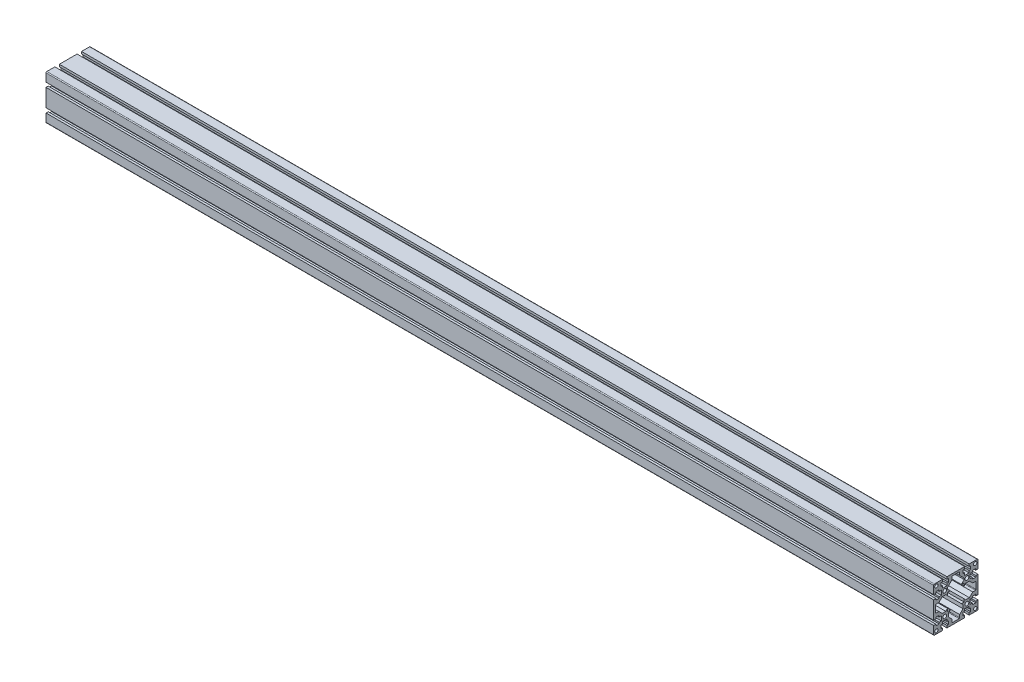
SolidWorks part; units mm, degrees
ref_plane "Front Plane" through (0, 0, 0) normal (0, 0, 1) x (1, 0, 0)
ref_plane "Top Plane" through (0, 0, 0) normal (0, 1, 0) x (1, 0, 0)
ref_plane "Right Plane" through (0, 0, 0) normal (1, 0, 0) x (0, 0, -1)
sketch "草图1" plane through (0, 0, 0) normal (0, 0, 1) x (1, 0, 0)
  line L0 (-530.3448, 0) -> (1069.6552, 0)
  dimension "D1" = 1600
other "Aluminum profile 80 X 80G X R1.5(1)"
ref_plane "Plane2" through (-530.3448, 0, 0) normal (1, 0, 0) x (0, 1, 0)
sketch "Sketch1" plane through (-530.3448, 0, 0) normal (1, 0, 0) x (0, 1, 0)
  line L0 (0, 40) -> (0, 0) construction
  line L1 (0, 0) -> (40, 0) construction
  line L2 (-24.05, 40) -> (-24.05, 36)
  line L3 (-38.5, 40) -> (-24.05, 40)
  line L4 (-40, 38.5) -> (-40, 24.05)
  line L5 (-38.5, -40) -> (-24.05, -40)
  line L6 (40, 38.5) -> (40, 24.05)
  line L7 (-24.05, 36) -> (-26.75, 36)
  line L8 (-26.75, 36) -> (-26.75, 30)
  line L9 (-26.75, 30) -> (-24.05, 30)
  line L10 (-24.05, 30) -> (-24.05, 26)
  line L11 (-24.05, 26) -> (-15.95, 26)
  line L12 (-15.95, 26) -> (-15.95, 30)
  line L13 (-15.95, 30) -> (-13.25, 30)
  line L14 (-13.25, 30) -> (-13.25, 36)
  line L15 (-13.25, 36) -> (-15.95, 36)
  line L16 (-15.95, 36) -> (-15.95, 40)
  line L17 (-40, 15.95) -> (-36, 15.95)
  line L18 (-36, 15.95) -> (-36, 13.25)
  line L19 (-15.95, 40) -> (15.95, 40)
  line L20 (-20, 20) -> (-20, 40) construction
  line L21 (20, 20) -> (20, 40) construction
  line L22 (15.95, 36) -> (15.95, 40)
  line L23 (13.25, 36) -> (15.95, 36)
  line L24 (13.25, 30) -> (13.25, 36)
  line L25 (15.95, 30) -> (13.25, 30)
  line L26 (-36, 13.25) -> (-30, 13.25)
  line L27 (-30, 13.25) -> (-30, 15.95)
  line L28 (-26, 15.95) -> (-26, 24.05)
  line L29 (-26, 24.05) -> (-30, 24.05)
  line L30 (-30, 24.05) -> (-30, 26.75)
  line L31 (-30, 26.75) -> (-36, 26.75)
  line L32 (-36, 26.75) -> (-36, 24.05)
  line L33 (-36, 24.05) -> (-40, 24.05)
  line L34 (-30, 15.95) -> (-26, 15.95)
  line L35 (15.95, 26) -> (15.95, 30)
  line L36 (24.05, 26) -> (15.95, 26)
  line L37 (24.05, 30) -> (24.05, 26)
  line L38 (26.75, 30) -> (24.05, 30)
  line L39 (26.75, 36) -> (26.75, 30)
  line L40 (24.05, 36) -> (26.75, 36)
  line L41 (24.05, 40) -> (24.05, 36)
  line L42 (24.05, -40) -> (24.05, -36)
  line L43 (24.05, -36) -> (26.75, -36)
  line L44 (26.75, -36) -> (26.75, -30)
  line L45 (26.75, -30) -> (24.05, -30)
  line L46 (24.05, -30) -> (24.05, -26)
  line L47 (24.05, -26) -> (15.95, -26)
  line L48 (15.95, -26) -> (15.95, -30)
  line L49 (15.95, -30) -> (13.25, -30)
  line L50 (13.25, -30) -> (13.25, -36)
  line L51 (13.25, -36) -> (15.95, -36)
  line L52 (15.95, -36) -> (15.95, -40)
  line L53 (-15.95, -36) -> (-15.95, -40)
  line L54 (-13.25, -36) -> (-15.95, -36)
  line L55 (-13.25, -30) -> (-13.25, -36)
  line L56 (-15.95, -30) -> (-13.25, -30)
  line L57 (-15.95, -26) -> (-15.95, -30)
  line L58 (-24.05, -26) -> (-15.95, -26)
  line L59 (-24.05, -30) -> (-24.05, -26)
  line L60 (-26.75, -30) -> (-24.05, -30)
  line L61 (-26.75, -36) -> (-26.75, -30)
  line L62 (-24.05, -36) -> (-26.75, -36)
  line L63 (-24.05, -40) -> (-24.05, -36)
  line L64 (-30, -15.95) -> (-26, -15.95)
  line L65 (-36, -26.75) -> (-36, -24.05)
  line L66 (-30, -26.75) -> (-36, -26.75)
  line L67 (-30, -24.05) -> (-30, -26.75)
  line L68 (-26, -24.05) -> (-30, -24.05)
  line L69 (-26, -15.95) -> (-26, -24.05)
  line L70 (-30, -13.25) -> (-30, -15.95)
  line L71 (-36, -13.25) -> (-30, -13.25)
  line L72 (-36, -15.95) -> (-36, -13.25)
  line L73 (36, 24.05) -> (40, 24.05)
  line L74 (40, 15.95) -> (36, 15.95)
  line L75 (36, -15.95) -> (36, -13.25)
  line L76 (36, -13.25) -> (30, -13.25)
  line L77 (30, -13.25) -> (30, -15.95)
  line L78 (26, -15.95) -> (26, -24.05)
  line L79 (26, -24.05) -> (30, -24.05)
  line L80 (30, -24.05) -> (30, -26.75)
  line L81 (30, -26.75) -> (36, -26.75)
  line L82 (36, -26.75) -> (36, -24.05)
  line L83 (30, -15.95) -> (26, -15.95)
  line L84 (30, 15.95) -> (26, 15.95)
  line L85 (36, 26.75) -> (36, 24.05)
  line L86 (30, 26.75) -> (36, 26.75)
  line L87 (30, 24.05) -> (30, 26.75)
  line L88 (26, 24.05) -> (30, 24.05)
  line L89 (26, 15.95) -> (26, 24.05)
  line L90 (30, 13.25) -> (30, 15.95)
  line L91 (36, 13.25) -> (30, 13.25)
  line L92 (36, 15.95) -> (36, 13.25)
  line L93 (-36, -15.95) -> (-40, -15.95)
  line L94 (-36, -24.05) -> (-40, -24.05)
  line L95 (36, -15.95) -> (40, -15.95)
  line L96 (36, -24.05) -> (40, -24.05)
  line L97 (-13, 18) -> (-10, 15)
  line L98 (-15, 15) -> (-10, 15)
  line L99 (-15, 15) -> (-15, 10)
  line L100 (-15, -15) -> (-10, -15)
  line L101 (15, 15) -> (15, 10)
  line L102 (-18, 13) -> (-15, 10)
  line L104 (13, 18) -> (10, 15)
  line L105 (13, -18) -> (10, -15)
  line L106 (20, -15) -> (15, -10)
  line L107 (-18, -13) -> (-15, -10)
  line L108 (-13, -18) -> (-10, -15)
  line L109 (15, -10) -> (15, -15)
  line L110 (10, 15) -> (15, 15)
  line L111 (-15, -10) -> (-15, -15)
  line L112 (10, -15) -> (15, -15)
  line L113 (15, 10) -> (20, 15)
  line L235 (24.05, 40) -> (38.5, 40)
  line L249 (-40, 15.95) -> (-40, -15.95)
  line L250 (-20, 20) -> (-26, 20) construction
  line L264 (40, 15.95) -> (40, -15.95)
  line L265 (-13, 24.5) -> (-7, 30.5)
  line L266 (-7, 30.5) -> (-7, 35.5)
  line L267 (7, 35.5) -> (7, 30.5)
  line L268 (7, 30.5) -> (13, 24.5)
  line L269 (-6, -36.5) -> (6, -36.5)
  line L270 (-13, 24.5) -> (-13, 18)
  line L271 (-35.5, 7) -> (-30.5, 7)
  line L272 (-30.5, 7) -> (-24.5, 13)
  line L273 (-24.5, 13) -> (-18, 13)
  line L274 (13, 24.5) -> (13, 18)
  line L275 (-15.95, -40) -> (15.95, -40)
  line L276 (35.5, 7) -> (30.5, 7)
  line L277 (30.5, 7) -> (22.5, 15)
  line L278 (24.05, -40) -> (38.5, -40)
  line L279 (20, 15) -> (22.5, 15)
  line L333 (-13, -24.5) -> (-13, -18)
  line L336 (-13, -24.5) -> (-7, -30.5)
  line L385 (-7, -30.5) -> (-7, -35.5)
  line L386 (-36.5, 6) -> (-36.5, -6)
  line L387 (7, -35.5) -> (7, -30.5)
  line L429 (7, -30.5) -> (13, -24.5)
  line L430 (13, -24.5) -> (13, -18)
  line L494 (20, -15) -> (22.5, -15)
  line L496 (30.5, -7) -> (22.5, -15)
  line L497 (35.5, -7) -> (30.5, -7)
  line L498 (-24.5, -13) -> (-18, -13)
  line L499 (-30.5, -7) -> (-24.5, -13)
  line L500 (-35.5, -7) -> (-30.5, -7)
  line L512 (40, -24.05) -> (40, -38.5)
  line L519 (-40, -24.05) -> (-40, -38.5)
  line L520 (-6, 36.5) -> (6, 36.5)
  line L523 (36.5, 6) -> (36.5, -6)
  circle A0 centre (-20, 20) radius 3.4
  circle A2 centre (20, 20) radius 3.4
  circle A3 centre (20, -20) radius 3.4
  circle A7 centre (-20, -20) radius 3.4
  arc A8 (-38.5, 40) -> (-40, 38.5) centre (-38.5, 38.5) ccw
  arc A9 (-40, -38.5) -> (-38.5, -40) centre (-38.5, -38.5) ccw
  arc A10 (38.5, -40) -> (40, -38.5) centre (38.5, -38.5) ccw
  arc A11 (38.5, 40) -> (40, 38.5) centre (38.5, 38.5) cw
  circle A12 centre (-35, 35) radius 3
  circle A13 centre (35, 35) radius 3
  circle A14 centre (35, -35) radius 3
  arc A15 (-6, 36.5) -> (-7, 35.5) centre (-6, 35.5) ccw
  arc A16 (6, 36.5) -> (7, 35.5) centre (6, 35.5) cw
  arc A17 (-36.5, 6) -> (-35.5, 7) centre (-35.5, 6) cw
  arc A18 (-36.5, -6) -> (-35.5, -7) centre (-35.5, -6) ccw
  arc A19 (36.5, -6) -> (35.5, -7) centre (35.5, -6) cw
  arc A20 (36.5, 6) -> (35.5, 7) centre (35.5, 6) ccw
  arc A21 (6, -36.5) -> (7, -35.5) centre (6, -35.5) ccw
  arc A22 (-6, -36.5) -> (-7, -35.5) centre (-6, -35.5) cw
  point P48 (-20, 20)
  point P97 (0, 0)
  point P104 (-7, 36.5)
  point P185 (40, 40)
  point P187 (40, -40)
  point P188 (-40, -40)
  point P190 (-40, 40)
  dimension "D1" = 80
  dimension "D2" = 80
  dimension "D3" = 20
  dimension "D4" = 8.1
  dimension "D5" = 45
  dimension "D6" = 7
  dimension "D7" = 13.5
  dimension "D8" = 6
  dimension "D12" = 5
  dimension "D13" = 5
  dimension "D14" = 20
  dimension "D18" = 1
  dimension "D19" = 14
  dimension "D15" = 6.8
  dimension "D27" = 45
  dimension "D20" = 1.5
  dimension "D11" = 6
  dimension "D9" = 4
  dimension "D10" = 14
  dimension "D16" = 14
  dimension "D17" = 45
  dimension "D21" = 3.5
  dimension "D22" = 3.5
  dimension "D23" = 73
  dimension "D24" = 30
  dimension "D25" = 30
  dimension "D26" = 45
  dimension "D28" = 5
sketch "Sketch10" plane through (1069.6552, 0, 0) normal (1, 0, 0) x (0, 0, -1)
  circle A0 centre (35, -35) radius 3
  circle A1 centre (-35, -35) radius 3 construction
  circle A2 centre (35, 35) radius 3 construction
  dimension "D1" = 6
  dimension "D2" = 70
  dimension "D3" = 70
extrude "Cut-Extrude1" cut sketch "Sketch10" against normal through all
